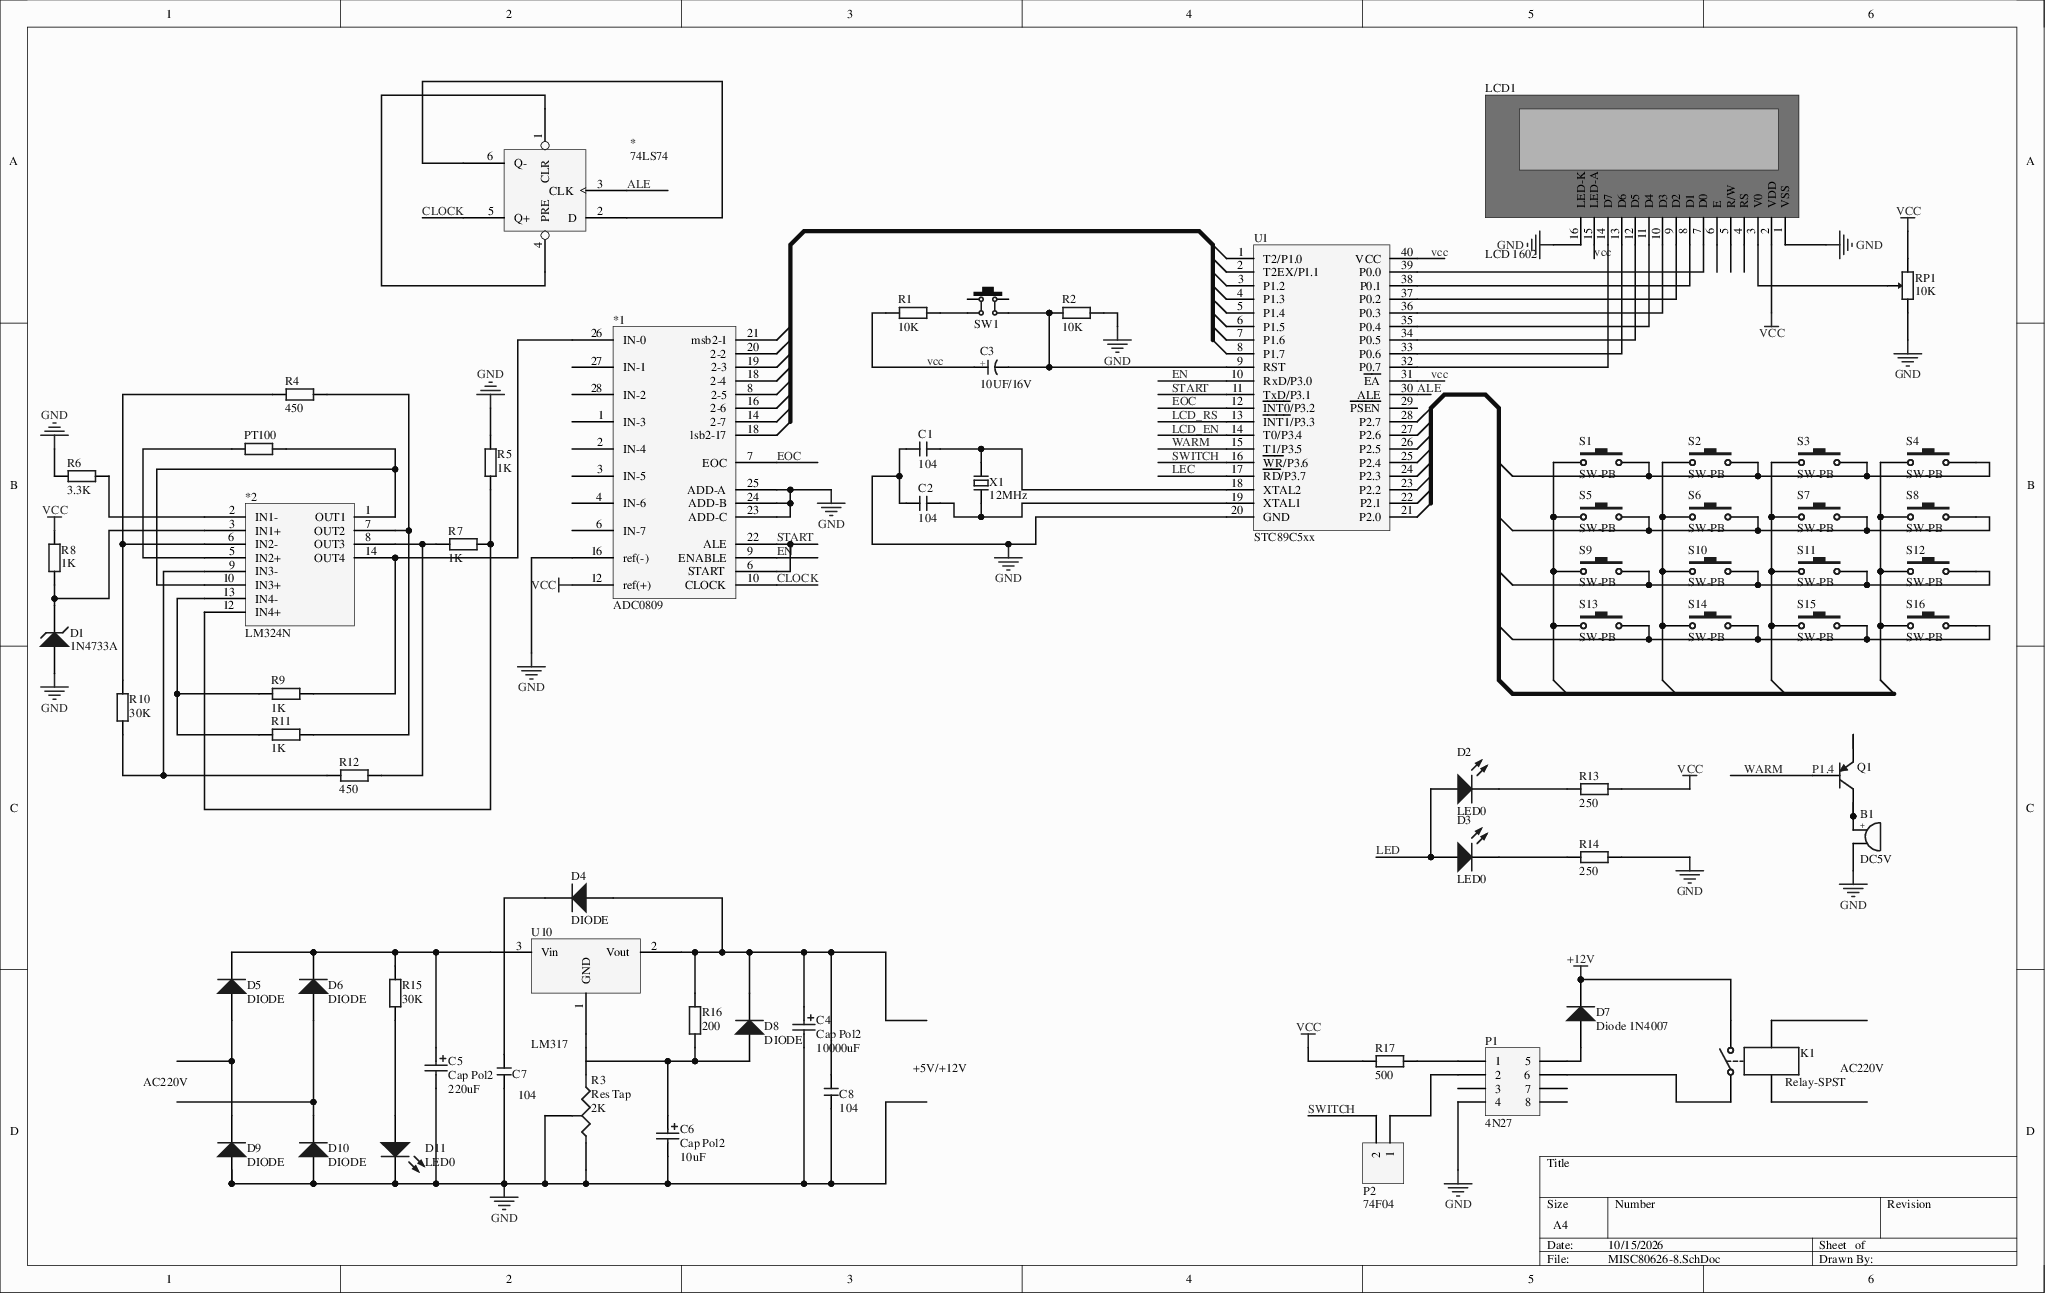
[diagram p0: MISC80626-8.SchDoc]
# Altium project MISC80626-9.PrjPcb
1 sheet, 67 parts. Net scope: global (net labels, ports and power ports of the same name join across sheets).
Board file: MISC80626.PcbDoc

## Sheet MISC80626-8.SchDoc
size 381 x 241 mm

### Parts
*  74LS74  [646-06]
*1  ADC0809  [N28B]
*2  LM324N  [646-06]
B1  DC5V  [PIN2]
C1  104  [RAD-0.3]
C2  104  [RAD-0.3]
C3  10UF/16V  [RB7.6-15]
C4  Cap Pol2  value 10000uF  [POLAR0.8]
C5  Cap Pol2  value 220uF  [POLAR0.8]
C6  Cap Pol2  value 10uF  [POLAR0.8]
C7  104  [RAD-0.3]
C8  104  [RAD-0.3]
D1  1N4733A  [DIODE-0.7]
D2  LED0  [LED-0]
D3  LED0  [LED-0]
D4  DIODE  [DO-201AD]
D5  DIODE  [DO-201AD]
D6  DIODE  [DO-201AD]
D7  Diode 1N4007  [DO-41]
D8  DIODE  [DO-201AD]
D9  DIODE  [DO-201AD]
D10  DIODE  [DO-201AD]
D11  LED0  [LED-0]
K1  Relay-SPST  [MODULE4]
LCD1  LCD 1602  [LCD1602]
P1  4N27  [HDR2X4]
P2  74F04  [HDR1X2]
PT100  30K  [AXIAL-0.4]  (value not drawn)
Q1  2N3906  [TO-92A]  (value not drawn)
R1  10K  [AXIAL-0.4]
R2  10K  [AXIAL-0.4]
R3  Res Tap  value 2K  [VR3]
R4  450  [AXIAL-0.4]
R5  1K  [AXIAL-0.4]
R6  3.3K  [AXIAL-0.4]
R7  1K  [AXIAL-0.4]
R8  1K  [AXIAL-0.4]
R9  1K  [AXIAL-0.4]
R10  30K  [AXIAL-0.4]
R11  1K  [AXIAL-0.4]
R12  450  [AXIAL-0.4]
R13  250  [AXIAL-0.4]
R14  250  [AXIAL-0.4]
R15  30K  [AXIAL-0.4]
R16  200  [AXIAL-0.4]
R17  500  [AXIAL-0.4]
RP1  10K  [电位器]
S1  SW-PB  [SPST-2]
S2  SW-PB  [SPST-2]
S3  SW-PB  [SPST-2]
S4  SW-PB  [SPST-2]
S5  SW-PB  [SPST-2]
S6  SW-PB  [SPST-2]
S7  SW-PB  [SPST-2]
S8  SW-PB  [SPST-2]
S9  SW-PB  [SPST-2]
S10  SW-PB  [SPST-2]
S11  SW-PB  [SPST-2]
S12  SW-PB  [SPST-2]
S13  SW-PB  [SPST-2]
S14  SW-PB  [SPST-2]
S15  SW-PB  [SPST-2]
S16  SW-PB  [SPST-2]
SW1  6x6x5  [四脚轻触开关]  (value not drawn)
U1  STC89C5xx  [DIP40]
U10  LM317  [TO220A]
X1  12MHz  [R38]

### Nets
+12V: D7.2(K) K1.2
GND: *1.16(2-6) *1.23(ADD-C) *1.24(ADD-B) *1.25(ADD-A) B1.2 C1.1 C2.1 C4.2 C5.2 C6.2 C7.1 C8.1 D1.1(A) D9.1(A) D10.1(A) D11.2(K) LCD1.1(VSS) LCD1.16(LED-K) P1.4 R2.2 R3.1(A) R3.3(TAP) R5.1 R6.2 R14.2 RP1.1 U1.20(GND)
vcc: *1.12(ref(+)) C3.1(A) LCD1.2(VDD) LCD1.15(LED-A) R1.1 R8.2 R13.2 R17.1 RP1.3 U1.31(~{EA}) U1.40(VCC)
ALE: *.3(CLK) U1.30(ALE)
CLOCK: *.5(Q+) *1.10(CLOCK)
EN: *1.9(ENABLE) U1.10(RxD/P3.0)
EOC: *1.7(EOC) U1.12(~{INT0}/P3.2)
LCD_EN: U1.14(T0/P3.4)
LCD_RS: U1.13(~{INT1}/P3.3)
LEC: U1.17(~{RD}/P3.7)
LED: D2.1(A) D3.1(A)
P1.4: Q1.2(B) U1.15(T1/P3.5)  [also labelled WARM]
START: *1.6(START) *1.22(ALE) U1.11(TxD/P3.1)
SWITCH: P2.2 U1.16(~{WR}/P3.6)
Net*1_26: *1.26(IN-0) *2.14(OUT4) R9.1
Net*2_1: *2.1(OUT1) *2.10(IN3+) PT100.1
Net*2_2: *2.2(IN1-) R6.1
Net*2_3: *2.3(IN1+) D1.2(K) R8.1
Net*2_5: *2.5(IN2+) PT100.2
Net*2_6: *2.6(IN2-) R4.2 R10.1
Net*2_7: *2.7(OUT2) R4.1 R11.1
Net*2_8: *2.8(OUT3) R7.2 R12.1
Net*2_9: *2.9(IN3-) R10.2 R12.2
Net*2_12: *2.12(IN4+) R5.2 R7.1
Net*2_13: *2.13(IN4-) R9.2 R11.2
Net*_1: *.1(CLR) *.4(PRE)
Net*_2: *.2(D) *.6(Q-)
NetB1_1: B1.1 Q1.3(C)
NetC1_2: C1.2 U1.18(XTAL2) X1.2
NetC2_2: C2.2 U1.19(XTAL1) X1.1
NetC3_2: C3.2(K) R2.1 SW1.3 U1.9(RST)
NetC4_1: C4.1 C8.2 D4.1(A) D8.2(K) R16.2 U10.2(Vout)
NetC5_1: C5.1 D5.2(K) D6.2(K) R15.2 U10.3(Vin)
NetC6_1: C6.1 D8.1(A) R16.1
NetC7_2: C7.2 D4.2(K)
NetD2_2: D2.2(K) R13.1
NetD3_2: D3.2(K) R14.1
NetD5_1: D5.1(A) D9.2(K)
NetD6_1: D6.1(A) D10.2(K)
NetD7_1: D7.1(A) P1.5
NetD11_1: D11.1(A) R15.1
NetK1_1: K1.1 P1.6
NetLCD1_3: LCD1.3(V0) RP1.2
NetLCD1_7: LCD1.7(D0) U1.39(P0.0)
NetLCD1_8: LCD1.8(D1) U1.38(P0.1)
NetLCD1_9: LCD1.9(D2) U1.37(P0.2)
NetLCD1_10: LCD1.10(D3) U1.36(P0.3)
NetLCD1_11: LCD1.11(D4) U1.35(P0.4)
NetLCD1_12: LCD1.12(D5) U1.34(P0.5)
NetLCD1_13: LCD1.13(D6) U1.33(P0.6)
NetLCD1_14: LCD1.14(D7) U1.32(P0.7)
NetP1_1: P1.1 R17.2
NetP1_2: P1.2 P2.1
NetR1_2: R1.2 SW1.4
NetR3_2: R3.2(B) U10.1(GND)
NetS1_1: S1.1 S5.1 S9.1 S13.1
NetS1_2: S1.2 S2.2 S3.2 S4.2
NetS2_1: S2.1 S6.1 S10.1 S14.1
NetS3_1: S3.1 S7.1 S11.1 S15.1
NetS4_1: S4.1 S8.1 S12.1 S16.1
NetS5_2: S5.2 S6.2 S7.2 S8.2
NetS9_2: S9.2 S10.2 S11.2 S12.2
NetS13_2: S13.2 S14.2 S15.2 S16.2

Not connected (* = marked no-connect by the designer): *1 1(IN-3) 2(IN-4) 3(IN-5) 4(IN-6) 8(2-5) 14(2-7) 18(2-4) 19(2-3) 20(2-2) 21(msb2-1) 27(IN-1) 28(IN-2); K1 3 4; LCD1 4(RS) 5(R/W) 6(E); P1 3 7 8; Q1 1(E); SW1 1 2; U1 1(T2/P1.0) 2(T2EX/P1.1) 3(P1.2) 4(P1.3) 5(P1.4) 6(P1.5) 7(P1.6) 8(P1.7) 21(P2.0) 22(P2.1) 23(P2.2) 24(P2.3) 25(P2.4) 26(P2.5) 27(P2.6) 28(P2.7) 29(~{PSEN})

### Notes on the sheet
- AC220V
- +5V/+12V

### Library data of the parts
* *1 *2 = Component_1
B1 = BEEP: Buzzer; 版权归属: COMPANY_A; BOM名称: Buzzer
C1 C2 C7 C8 = C-CC: Through-hole ceramic capacitor; 版权归属: COMPANY_A; BOM名称: Through-hole ceramic capacitor
C3 = C-CAP: Through-hole electrolytic capacitor; 版权归属: COMPANY_A; BOM名称: Through-hole electrolytic capacitor
C4-C6 = Cap Pol2: Polarized Capacitor (Axial); Published: 8-Jun-2000; LatestRevisionDate: 17-Jul-2002; LatestRevisionNote: Re-released for DXP Platform.; PackageReference: POLAR0.8; Publisher: Altium Limited
D1 = D Zener: Zener Diode; Published: 8-Jun-2000; LatestRevisionDate: 17-Jul-2002; LatestRevisionNote: Re-released for DXP Platform.; PackageReference: DIODE-0.7; Publisher: Altium Limited
D2 D3 D11 = LED0: Typical INFRARED GaAs LED; Published: 8-Jun-2000; LatestRevisionDate: 08-Jul-2005; LatestRevisionNote: Mech Layer 1 removed.; PackageReference: LED-0; Publisher: Altium Limited
D4-D10 = Diode 1N5400: 3 Amp General Purpose Rectifier; Published: 8-Jun-2000; LatestRevisionDate: 17-Jul-2002; LatestRevisionNote: Re-released for DXP Platform.; DatasheetDocument: 1998; PackageDocument: Aug-1999; PackageReference: DO-201AD; ComponentLink1Description: Manufacturer Link; ComponentLink2Description: Datasheet; ComponentLink2URL: http://www.fairchildsemi.com/ds/1N%2F1N5400.pdf; Publisher: Altium Limited
K1 = Relay-SPST: Single-Pole Single-Throw Relay; Published: 24-Mar-1999; LatestRevisionDate: 17-Jul-2002; LatestRevisionNote: Re-released for DXP Platform.; PackageReference: MODULE4; Publisher: Altium Limited
LCD1 = LCD 1602: 版权归属: COMPANY_A; BOM名称: LCD 1602
P1 = Header 4X2A: Header, 4-Pin, Dual row; LatestRevisionDate: 17-Jul-2002; LatestRevisionNote: Re-released for DXP Platform.; Publisher: Altium Limited
P2 = Header 2: Header, 2-Pin; LatestRevisionDate: 17-Jul-2002; LatestRevisionNote: Re-released for DXP Platform.; Publisher: Altium Limited
PT100 R1 R2 R4-R17 = R-CRR: Through-hole colour-band resistor; 版权归属: COMPANY_A; BOM名称: Colour-band resistor
Q1 = 2N3906: PNP General Purpose Amplifier; Published: 8-Jun-2000; LatestRevisionDate: 15-Jan-2003; LatestRevisionNote: PCB Footprint 'BCY-W3/D4.7' replaced; DatasheetDocument: 1997; PackageDocument: Sep-1998; PackageReference: TO-92A; Code_JEDEC: TO-92A; ComponentLink1Description: Manufacturer Link; ComponentLink2Description: Datasheet; ComponentLink2URL: http://www.fairchildsemi.com/ds/2N%2F2N3906.pdf; Publisher: Altium Limited
R3 = Res Tap: Tapped Resistor; Sim Note: Enter the Resistance value and the set point into parameter fields.; Set Position: 0.5; Published: 24-Mar-1999; LatestRevisionDate: 17-Jul-2002; LatestRevisionNote: Re-released for DXP Platform.; PackageReference: VR3; Publisher: Altium Limited
RP1 = RP-ID: Plug-in single-gang potentiometer; BOM名称: Plug-in potentiometer; 版权归属: COMPANY_A
S1-S16 = SW-PB: Switch; Published: 24-Mar-1999; LatestRevisionDate: 17-Jul-2002; LatestRevisionNote: Re-released for DXP Platform.; PackageReference: SPST-2; Publisher: Altium Limited
SW1 = TSW DIP-6x6: Through-hole 6x6 tactile switch; 版权归属: COMPANY_A; BOM名称: Through-hole 6x6 tactile switch
U1 = STC89C5xx: STC microcontroller; 版权归属: COMPANY_A; BOM名称: STC microcontroller
U10 = LM317: Adjustable linear regulator IC
X1 = XTAL-2: 2-pin crystal oscillator; 版权归属: COMPANY_A; BOM名称: 2-pin crystal oscillator